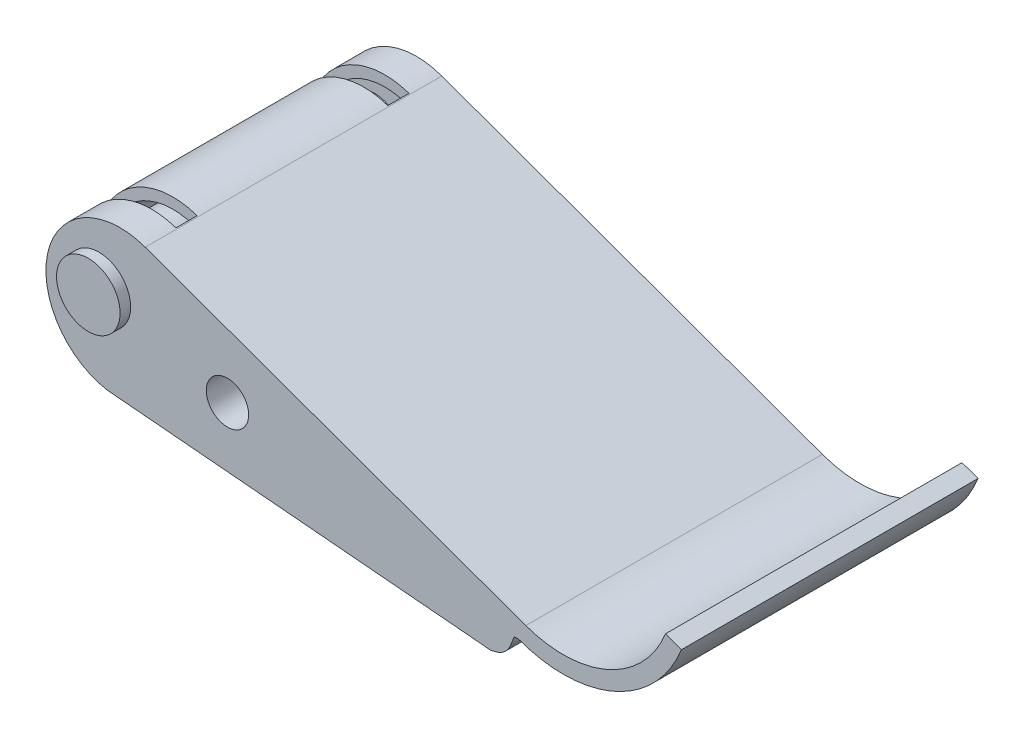
from build123d import *

# Parameters (mm, degrees)
EXTRUDE_1_DEPTH          = 7
EXTRUDE_1_DEPTH_BACK     = 7
SKETCH_1_R               = 1
CUT_EXTRUDE_1_DEPTH      = 6
CUT_EXTRUDE_1_DEPTH_BACK = 6
CUT_EXTRUDE_2_DEPTH      = 6
CUT_EXTRUDE_2_DEPTH_BACK = 6
SKETCH_3_R               = 3
CUT_EXTRUDE_START        = -1
CUT_EXTRUDE_3_DEPTH      = 1
CUT_EXTRUDE_4_DEPTH      = 1
EXTRUDE_2_DEPTH          = 7.5
EXTRUDE_2_DEPTH_BACK     = 7.5
SKETCH_6_R               = 1.5
CUT_EXTRUDE_5_DEPTH      = 5.5
CUT_EXTRUDE_5_DEPTH_BACK = 5.5


with BuildPart() as part:
    # 草图1 → 凸台-拉伸1 (new, two sides: drawn at the far end of the back side and taken through both)
    with BuildSketch(Plane.XY.offset(-EXTRUDE_1_DEPTH_BACK)):
        with BuildLine():
            Line((2.892231378, 2.053172864), (21, 0.468948388))
            Line((21, 0.468948388), (21.243569075, 0.530116447))
            ThreePointArc((21.243569075, 0.530116447), (21.657311704, 0.746381181), (21.927791013, 1.126899697))
            Line((21.927791013, 1.126899697), (22.11, 1.58))
            Line((22.11, 1.58), (22.31866709, 1.58))
            ThreePointArc((22.31866709, 1.58), (26.857258232, 1.7173207), (30, 4.994642886))
            Line((30, 4.994642886), (29.24792212, 5.268376848))
            ThreePointArc((29.24792212, 5.268376848), (26.549597889, 2.45607622), (22.654950899, 2.308721878))
            Line((22.654950899, 2.308721878), (4.688013818, 8.792206429))
            ThreePointArc((4.688013818, 8.792206429), (0.118016194, 6.401213367), (2.892231378, 2.053172864))
        make_face()
        with Locations((8.57, 4.38)):
            Circle(SKETCH_1_R, mode=Mode.SUBTRACT)
    extrude(amount=EXTRUDE_1_DEPTH + EXTRUDE_1_DEPTH_BACK)

    # 草图2 → 切除-拉伸1 (cut, two sides: drawn at the far end of the back side and taken through both)
    with BuildSketch(Plane.XY.offset(-CUT_EXTRUDE_1_DEPTH_BACK)):
        with BuildLine():
            Line((4.63, 0.629363491), (3.5, 5.5))
            Line((3.5, 5.5), (-1.5, 5.5))
            ThreePointArc((-1.5, 5.5), (0.389533797, 1.585284174), (4.63, 0.629363491))
        make_face()
    extrude(amount=CUT_EXTRUDE_1_DEPTH + CUT_EXTRUDE_1_DEPTH_BACK, mode=Mode.SUBTRACT)

    # 草图3 → 切除-拉伸2 (cut, two sides: drawn at the far end of the back side and taken through both)
    with BuildSketch(Plane.XY.offset(-CUT_EXTRUDE_2_DEPTH_BACK)):
        with Locations((3.5, 5.5)):
            Circle(SKETCH_3_R)
    extrude(amount=CUT_EXTRUDE_2_DEPTH + CUT_EXTRUDE_2_DEPTH_BACK, mode=Mode.SUBTRACT)

    # 草图4 → 切除-拉伸3 (cut)
    with BuildSketch(Plane.XY.offset(5.5).offset(CUT_EXTRUDE_START)):
        with BuildLine():
            Line((2.360511459, 2.190684985), (4.639488541, 8.809315015))
            ThreePointArc((4.639488541, 8.809315015), (0.190684985, 6.639488541), (2.360511459, 2.190684985))
        make_face()
    extrude(amount=CUT_EXTRUDE_3_DEPTH, mode=Mode.SUBTRACT)

    # 草图5 → 切除-拉伸4 (cut)
    with BuildSketch(Plane.XY.offset(-5.5)):
        with BuildLine():
            Line((2.360511459, 2.190684985), (4.639488541, 8.809315015))
            ThreePointArc((4.639488541, 8.809315015), (0.190684985, 6.639488541), (2.360511459, 2.190684985))
        make_face()
    extrude(amount=CUT_EXTRUDE_4_DEPTH, mode=Mode.SUBTRACT)

    # 草图6 → 凸台-拉伸2 (add, two sides: drawn at the far end of the back side and taken through both)
    with BuildSketch(Plane.XY.offset(-EXTRUDE_2_DEPTH_BACK)):
        with Locations((2.5, 6)):
            Circle(SKETCH_6_R)
    extrude(amount=EXTRUDE_2_DEPTH + EXTRUDE_2_DEPTH_BACK)

    # 草图7 → 切除-拉伸5 (cut, two sides: drawn at the far end of the back side and taken through both)
    with BuildSketch(Plane.XY.offset(-CUT_EXTRUDE_5_DEPTH_BACK)):
        Polygon((11.724964743, 1.0104331), (21.686911724, 0.138875672), (21.747920744, 0.836211961), (11.785973763, 1.707769388), align=None)
    extrude(amount=CUT_EXTRUDE_5_DEPTH + CUT_EXTRUDE_5_DEPTH_BACK, mode=Mode.SUBTRACT)


solid = part.part
